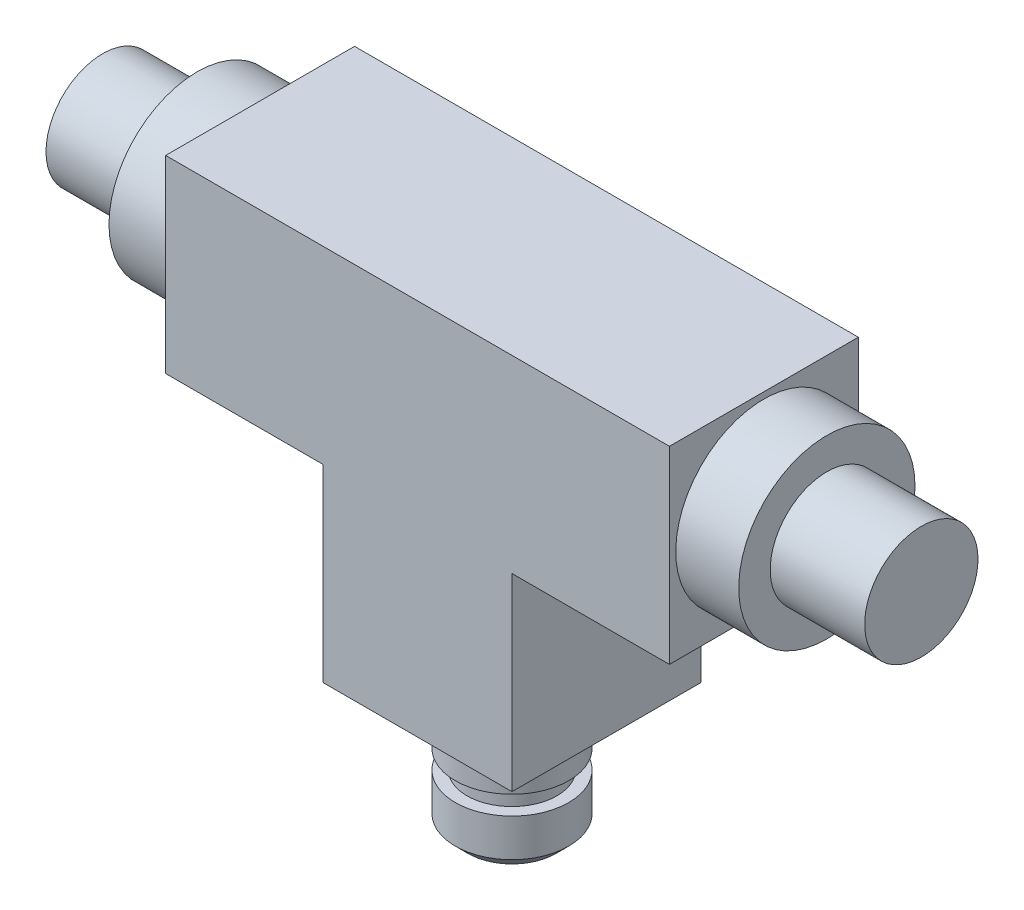
SolidWorks part; units mm, degrees
ref_plane "Front Plane" through (0, 0, 0) normal (0, 0, 1) x (1, 0, 0)
ref_plane "Top Plane" through (0, 0, 0) normal (0, 1, 0) x (1, 0, 0)
ref_plane "Right Plane" through (0, 0, 0) normal (1, 0, 0) x (0, 0, -1)
sketch "Sketch1" plane through (0, 0, 0) normal (0, 0, 1) x (1, 0, 0)
  line L0 (0, 0) -> (0, 30)
  line L1 (0, 30) -> (-25, 30)
  line L2 (-25, 30) -> (-25, 60)
  line L3 (-25, 60) -> (55, 60)
  line L4 (55, 60) -> (55, 30)
  line L5 (55, 30) -> (30, 30)
  line L6 (30, 30) -> (30, 0)
  line L7 (30, 0) -> (0, 0)
  dimension "D1" = 30
  dimension "D2" = 80
  dimension "D3" = 30
  dimension "D4" = 25
  dimension "D5" = 30
extrude "Boss-Extrude1" add sketch "Sketch1" along normal blind 30
sketch "Sketch2" plane through (55, 0, 0) normal (1, 0, 0) x (0, 0, -1)
  line L0 (-30, 30) -> (0, 30) construction
  circle A0 centre (-15, 45) radius 14
  dimension "D1" = 28
  dimension "D2" = 15
extrude "Boss-Extrude2" add sketch "Sketch2" along normal blind 10
sketch "Sketch3" plane through (65, 0, 0) normal (1, 0, 0) x (0, 0, -1)
  circle A0 centre (-15, 45) radius 9
  dimension "D1" = 18
extrude "Boss-Extrude3" add sketch "Sketch3" along normal blind 15
sketch "Sketch4" plane through (-25, 0, 0) normal (-1, 0, 0) x (0, 0, 1)
  line L0 (30, 30) -> (0, 30) construction
  circle A0 centre (15, 45) radius 14
  dimension "D1" = 28
  dimension "D2" = 15
extrude "Boss-Extrude4" add sketch "Sketch4" along normal blind 10
sketch "Sketch5" plane through (-35, 0, 0) normal (-1, 0, 0) x (0, 0, 1)
  circle A1 centre (15, 45) radius 9
  dimension "D2" = 18
extrude "Boss-Extrude5" add sketch "Sketch5" along normal blind 15
sketch "Sketch6" plane through (0, 0, 0) normal (0, -1, 0) x (-1, 0, 0)
  circle A0 centre (-15, -15) radius 9
  dimension "D1" = 18
extrude "Boss-Extrude6" add sketch "Sketch6" along normal blind 20
sketch "Sketch7" plane through (0, -20, 0) normal (0, -1, 0) x (-1, 0, 0)
  circle A0 centre (-15, -15) radius 7.148
  circle A1 centre (-15, -15) radius 10.2655
extrude "Cut-Extrude1" cut sketch "Sketch7" against normal blind 3 from offset 8 offset against normal yes
chamfer "Chamfer1" distance 2 angle 45 1 edges at (24, -20, 15)
sketch "Sketch8" plane through (0, 0, 0) normal (0, 0, -1) x (-1, 0, 0)
  circle A0 centre (-50, 45) radius 2.5
  circle A1 centre (20, 45) radius 2.5
extrude "Cut-Extrude2" cut sketch "Sketch8" against normal blind 6
